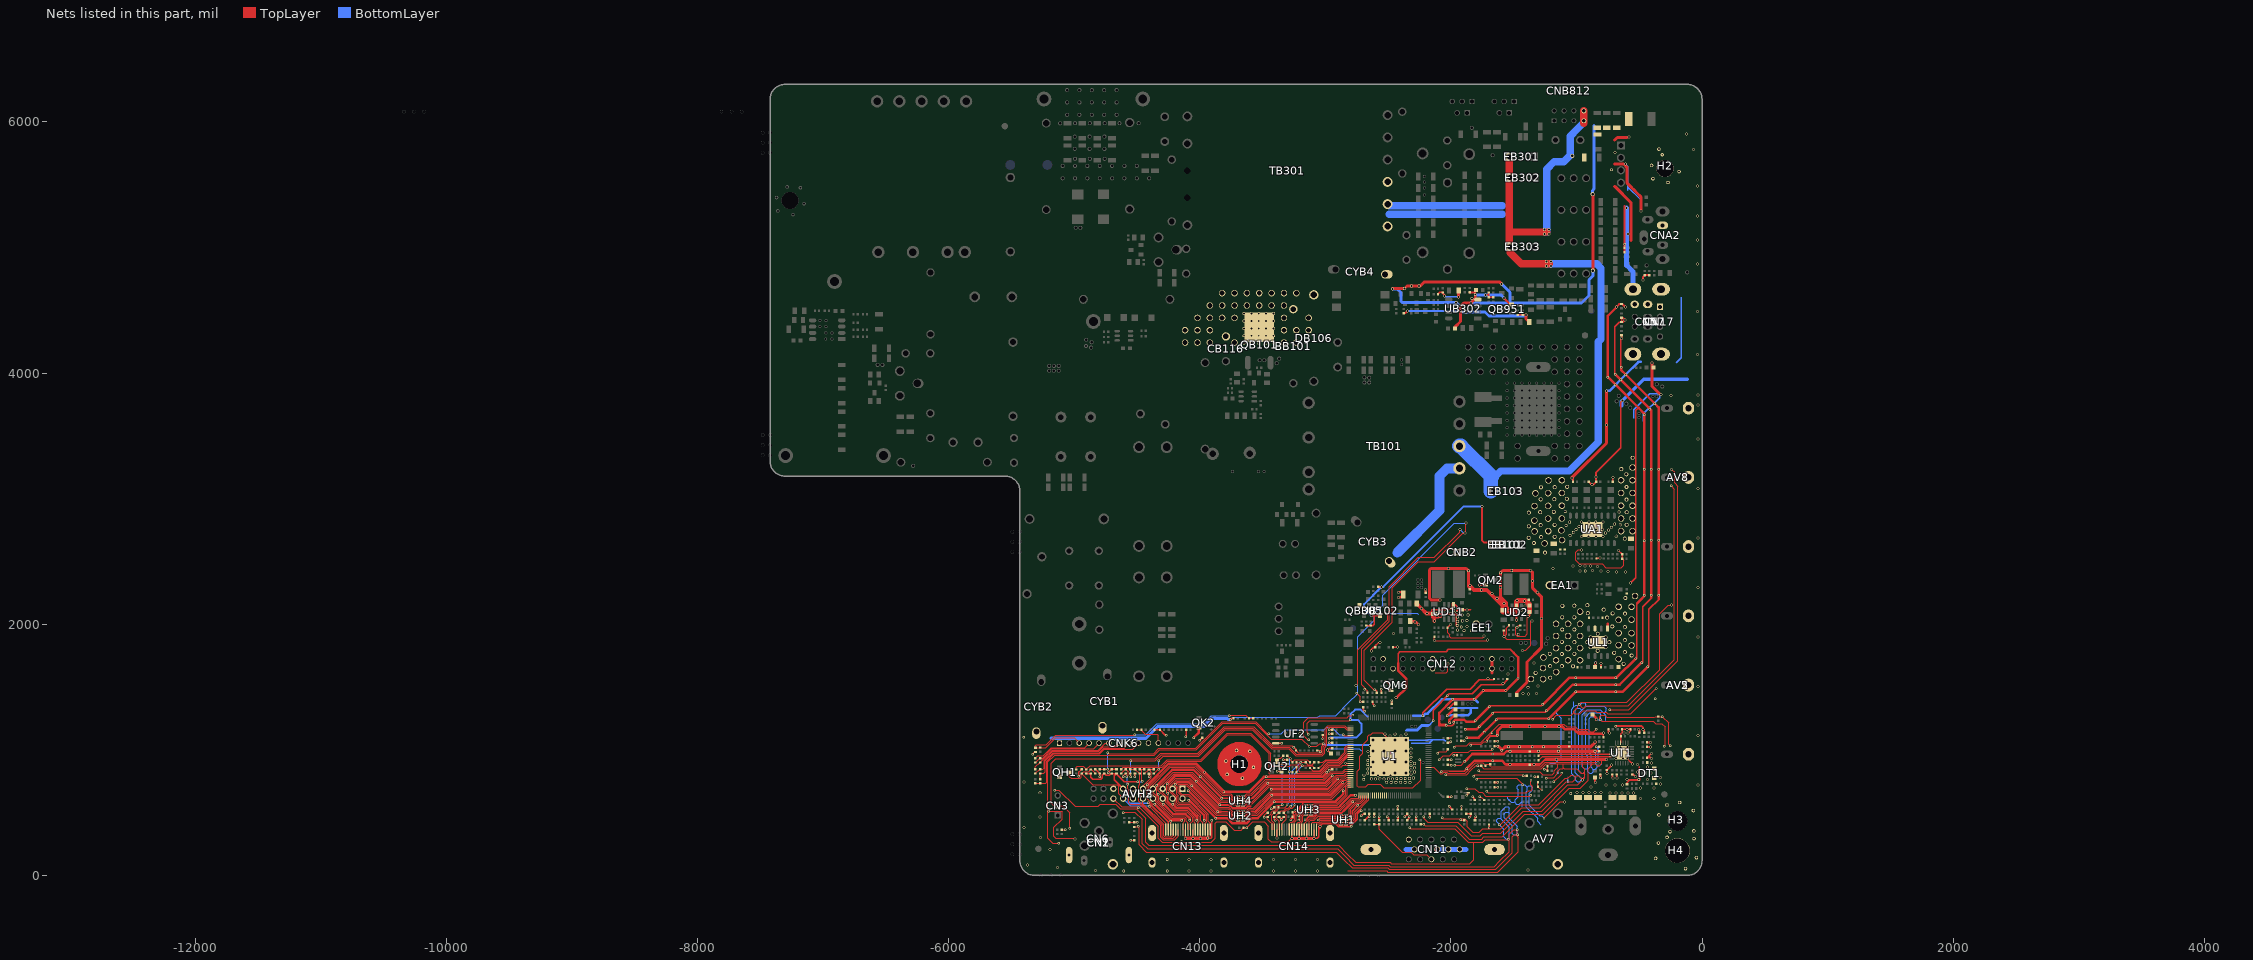
[diagram p0: the nets of this part, all layers, seen from the top]
# Altium PCB MISC84277.PcbDoc (part 10 of 15)
Units mil, origin at the board's own origin, x right, y up, seen from the top; angles counter-clockwise.
Board outline 7422.08 x 6299.21 mil, 2 copper layers (TopLayer, BottomLayer), stack 61.855 mil thick; 709 components, 395 nets, 2812 pads, 811 vias.

## Via types
v1: diameter 23.62, hole 15.75, TopLayer to BottomLayer, tented both sides, 437 vias
v2: diameter 19.68, hole 11.81, TopLayer to BottomLayer, tented both sides, 353 vias
v3: diameter 31.5, hole 23.62, TopLayer to BottomLayer, tented both sides, 16 vias
v4: diameter 31.5, hole 19.68, TopLayer to BottomLayer, tented both sides, 4 vias
v5: diameter 17.72, hole 9.84, TopLayer to BottomLayer, tented both sides, 1 vias

## Nets (pads, with @x,y where several pads share a name; then routed paths per layer and width w, separated by ;. In a path a pad name is that pad's centre, name@x,y a point inside that pad or via, vN(x,y) a via of type N, cw(c..) or ccw(c..) an arc to the next point about the centre after c; other vN are vias at no path point) (continued)
GND: (continued)
  other v1: -4606,34 -4259.5,34.5 -4085,34.5 -3910.5,34.5 -3413.04,34.5 -3238.54,34.5 -3064.04,34.5 -4829.1,37.25 -1387,41.5 -5132.2,62.6 -5372.8,82.7 -4259.5,124.5 -4085,124.5 -3910.5,124.5 -3413.04,124.5 -3238.54,124.5 -3064.04,124.5 -5194.2,204.1 -5268.5,300.8 -5400.94,382.6 -3043,388 -5271.8,463.9 -490.09,612.91 -382.59,612.91 -1046,652.26 -731.84,657.41 -685.09,657.41 -638.34,657.41 -591.59,657.41 -544.84,657.41 -5273.2,657.8 -994.84,658.91 -947.76,658.91 -900.67,658.91 -853.59,658.91 -806.5,658.91 -490.09,695.91 -382.59,695.91 -885,704.26 -33,718.5 -765.37,721.41 -694.12,721.41 -634.12,721.41 -330.5,727.76 -5400.94,743.7 -597.5,762.26 -435.12,763.41 -504.5,764.26 -332.5,777.76 -2582.1,795.6 -2482.7,796.2 -408.12,813.91 -513.5,824.76 -433.62,862.41 -1531,884.53 -1339,884.53 -513.12,884.41 -403.62,893.41 -1158,922.98 -685.18,930.04 -594.64,930.04 -628.9,931.02 -684.19,964.29 -595.63,986.33 -2662,987.1 -1302,988.47 -1142.5,988.47 -650.94,1019.59 -685.18,1020.59 -594.64,1020.59 -410.62,1021.41 -1541.4,1024.26 -1453.5,1024.26 -1352.5,1024.26 -1264.5,1024.26 -1140,1024.26 -2645.1,1034 -409.62,1059.41 -852.1,1063.1 -2399.4,1109.6 -2485.4,1110.4 -33,1112.2 -3204,1130 -3316,1134 -1526,1184.26 -1373,1184.26 -1252,1184.26 -841.6,1239.8 -1381,1445 -1426,1449 -1320,1450 -1386,1498 -33,1505.9 -1307,1509 -1585,1527 -1705,1568 -1544.11,1601.81 -1338,1691 -2634,1786 -33,1899.6 -1464,1917 -2458,1928 -1918,1979 -1872.05,1980.31 -1478,2033 -1280,2047 -1465,2082 -1504,2087 -2056,2088 -1951,2092 -1438,2108 -1532,2110 -1874,2115 -1409.26,2146.29 -1413.7,2184.95 -1474.71,2190.09 -1632.4,2204.1 -1672.2,2244.35 -1312.21,2251.54 -1758.7,2273.55 -1605,2292 -33,2293.3 -1352,2345 -682,2417 -611,2417 -748,2419 -930.5,2423.5 -973.3,2424.1 -806,2424 -872.9,2426.4 -1516,2428 -1187.1,2443.5 -833,2461 -932.9,2463.8 -1027,2465 -887.2,2465.6 -974,2466 -33,2687 -903,2697 -846,2697 -789,2697 -960,2699 -953.02,2754.94 -902.36,2754.94 -845.67,2754.94 -795.02,2754.94 -791,2813 -902,2814 -847,2814 -962,2815 -33,3080.7 -843.73,3171 -33,3474.41 -33,3747 -249,3823 -33,3824 -329,3829.5 -35.5,4146.5 -35.5,4489.5 -35.5,4868 -35.5,5059.25 -590.7,5108.6 -35.5,5250.5 -35.5,5491.5 -722.44,5619.47 -692.1,5758.6 -69,5779.5 -583.6,5881.4 -124,5906
  other v2: -4082.1,437.9 -3906.6,437.9 -4412.5,643.2 -4330.2,644.1 -4255.8,652.6 -4063.13,714.64 -1181,746 -4028.87,749.68 -3996.08,786.19 -3962.9,822.3 -1669,914.5 -1977,958 -1669,966.5 -3129.1,1026.27 -2971,1055 -1628,1069 -5400.94,1099.2 -2971,1127 -1735.14,1141.64 -1773.12,1184.27 -2038,1197 -1806,1233 -1694.53,1343.47 -373.4,1407.1 -689,1460.84 -2688,1482 -1007,1517.84 -689,1517.84 -1466.06,1570.27 -1007,1574.84 -689,1574.84 -433.33,1661.23 -481.87,1693.31 -528.64,1727.15 -2519,2088.94 -461,2230 -404,2230 -347,2230 -461,2666 -404,2667 -347,2667 -461,3236 -404,3236 -347,3236 -461,3670
  other v3: -2620.6,815.53 -2534.71,815.53 -2444.16,815.53 -2358.3,815.53 -2620.6,901.4 -2534.71,901.4 -2444.16,901.4 -2358.3,901.4 -2620.6,991.95 -2534.71,991.95 -2444.16,991.95 -2358.3,991.95 -2534.71,1077.82 -2444.16,1077.82
  other v4: -887.06,1816.63 -768.94,1816.63 -887.06,1895.37 -768.94,1895.37
H: BB101.1 CB116.2 DB106.A pad.VIA5@-3133.02,4341.45 pad.VIA5@-3133.02,4439.87 pad.VIA5@-3231.44,4243.02 pad.VIA5@-3231.44,4341.45 pad.VIA5@-3231.44,4636.72 pad.VIA5@-3329.86,4636.72 pad.VIA5@-3329.87,4243.02 pad.VIA5@-3329.87,4341.45 pad.VIA5@-3329.87,4439.87 pad.VIA5@-3329.87,4538.3 pad.VIA5@-3412.61,4238.33 pad.VIA5@-3412.61,4297.38 pad.VIA5@-3412.61,4356.44 pad.VIA5@-3412.61,4415.49 pad.VIA5@-3412.61,4474.55 pad.VIA5@-3428.29,4538.3 pad.VIA5@-3428.29,4636.72 pad.VIA5@-3471.66,4238.33 pad.VIA5@-3471.66,4297.38 pad.VIA5@-3471.66,4356.44 pad.VIA5@-3471.66,4415.49 pad.VIA5@-3471.66,4474.55 pad.VIA5@-3526.72,4538.3 pad.VIA5@-3526.72,4636.72 pad.VIA5@-3530.72,4238.33 pad.VIA5@-3530.72,4297.38 pad.VIA5@-3530.72,4356.44 pad.VIA5@-3530.72,4415.49 pad.VIA5@-3530.72,4474.55 pad.VIA5@-3589.77,4238.33 pad.VIA5@-3589.77,4297.38 pad.VIA5@-3589.77,4356.44 pad.VIA5@-3589.77,4415.49 pad.VIA5@-3589.77,4474.55 pad.VIA5@-3625.14,4538.3 pad.VIA5@-3625.14,4636.72 pad.VIA5@-3648.83,4238.33 pad.VIA5@-3648.83,4297.38 pad.VIA5@-3648.83,4356.44 pad.VIA5@-3648.83,4415.49 pad.VIA5@-3648.83,4474.55 pad.VIA5@-3723.57,4243.02 pad.VIA5@-3723.57,4439.87 pad.VIA5@-3723.57,4538.3 pad.VIA5@-3723.57,4636.72 pad.VIA5@-3821.99,4439.87 pad.VIA5@-3821.99,4538.3 pad.VIA5@-3821.99,4636.72 pad.VIA5@-3920.42,4243.02 pad.VIA5@-3920.42,4341.45 pad.VIA5@-3920.42,4439.87 pad.VIA5@-3920.42,4538.3 pad.VIA5@-4018.84,4243.02 pad.VIA5@-4018.84,4341.45 pad.VIA5@-4018.84,4439.88 pad.VIA5@-4117.27,4243.02 pad.VIA5@-4117.27,4341.45 QB101.D
HDMI1_5V: CH9.2 CN14.18 DH2.K RH8.2 RH9.2 RH14.2 RH15.1 | length 939.7
  TopLayer w8: CH9.2@-3412,498.73 -3412,495.03 -3426.84,480.19 -3426.84,434.84 -3405.51,413.51 CN14.18@-3405.51,398 ; CH9.2@-3408,498.73 -3402.75,498.73 -3376.6,524.88 -3376.6,537.97 DH2.K@-3373.17,541.4 ; CN14.18@-3405.51,364.62 CN14.18@-3405.51,398 ; CN14.18@-3405.51,411.51 CN14.18@-3405.51,398 ; DH2.K@-3369.27,538 -3325.26,538 -3317.74,545.52 -3317.68,545.52 -3305.8,557.4 v2(-3305.8,561.7) ; RH14.2@-3302.97,953.07 v2(-3277.9,928) -3277.9,915.8 RH9.2@-3263.03,899.9 -3242.49,920.44 -3143.51,920.44 RH8.2@-3122.97,899.9 ; v2(-3287.8,824) -3264.03,824 RH15.1@-3263.03,823
  BottomLayer w8: v2(-3305.8,561.7) -3282.47,585.03 -3282.47,796.2 ; -3282.47,807.47 -3282.47,796.2 ; v2(-3277.9,928) -3278.5,928 -3282.47,924.03 -3282.47,796.2
HDMI1_HPDIN: RH15.2 RH16.2 U1.113 | length 528.2
  TopLayer w6: RH15.2@-3235.27,823 -3225.1,812.84 -3036.51,812.84 -2971.35,878 -2885,878 -2824.2,938.8 U1.113@-2800.46,938.8 ; RH15.2@-3229.57,823 RH16.2@-3229.57,860
HDMI1_RX0_N: CN14.9 U1.1 UH3.3 UH3.6 | length 665.4
  TopLayer w7: CN14.9@-3228.35,364.62 -3228.35,408.29 -3214.3,422.34 -3205.76,422.34 -3192.84,435.26 -3192.84,475.03 -3166.46,501.41 UH3.3@-3154.64,501.41 UH3.6@-3113.7,501.41 -3098.06,501.41 -3074.14,525.34 -2885.26,525.34 -2795.59,615 -2738,615 -2733.53,619.47 U1.1@-2733.53,635.65
HDMI1_RX0_P: CN14.7 U1.2 UH3.4 UH3.5 | length 655.7
  TopLayer w7: CN14.7@-3188.98,364.62 -3190.53,366.17 -3190.53,420.6 -3180.84,430.29 -3180.84,470.06 -3169.17,481.73 UH3.4@-3154.64,481.73 UH3.5@-3113.7,481.73 -3100.78,481.73 -3069.17,513.34 -2880.29,513.34 -2790.62,603 -2726.54,603 -2717.79,611.76 U1.2@-2717.79,635.65
HDMI1_RX1_N: CN14.6 U1.3 UH1.1 UH1.8 | length 667
  TopLayer w7: CN14.6@-3168.04,364.62 -3168.04,409.54 -3125.56,452.03 -3092.3,452.03 -3062.99,481.34 -2937.1,481.34 ; -2912.7,481.34 -2937.1,481.34 ; UH1.1@-2878.24,481.34 -2937.1,481.34 ; UH1.1@-2875.97,480.67 UH1.8@-2835.03,480.67 -2820.13,480.67 -2811.7,489.1 -2811.7,529.6 -2754.3,587 -2722.97,587 -2702.04,607.93 U1.3@-2702.04,635.65
HDMI1_RX1_P: CN14.4 U1.4 UH1.2 UH1.7 | length 640.2
  TopLayer w7: CN14.4@-3128.67,364.62 -3128.67,429.36 -3118,440.03 -3087.33,440.03 -3058.02,469.34 -2901.07,469.34 -2892.72,460.98 UH1.2@-2875.97,460.98 UH1.7@-2835.03,460.98 -2822.84,460.98 -2799.7,484.13 -2799.7,524.63 -2749.33,575 -2718,575 -2686.29,606.71 U1.4@-2686.29,635.65
HDMI1_RX2_N: CN14.3 U1.5 UH1.3 UH1.6 | length 650.7
  TopLayer w7: CN14.3@-3108.99,364.62 -3108.99,414.65 -3101.31,422.34 -3050.56,422.34 -3035.56,437.34 -2925.2,437.34 ; -2912.7,437.34 -2925.2,437.34 ; U1.5@-2670.54,635.65 -2670.54,601.68 -2770.9,501.32 -2770.9,458.16 -2807.44,421.61 UH1.6@-2835.03,421.61 UH1.3@-2875.97,421.61 -2892.75,421.61 -2908.47,437.34 -2925.2,437.34
HDMI1_RX2_P: CN14.1 U1.6 UH1.4 UH1.5 | length 615.4
  TopLayer w7: CN14.1@-3069.62,364.62 -3069.62,403.97 -3063.25,410.34 -3045.59,410.34 -3030.59,425.34 -2913.44,425.34 -2890.04,401.93 UH1.4@-2875.97,401.93 UH1.5@-2835.03,401.93 -2822.09,401.93 -2814.4,409.61 -2802.47,409.61 -2758.9,453.19 -2758.9,496.35 -2654.79,600.46 U1.6@-2654.79,635.65
HDMI1_RXC_N: CN14.12 U1.127 UH3.1 UH3.8 | length 720.1
  TopLayer w7: CN14.12@-3286.15,364.62 -3286.15,413.85 -3277.35,422.65 -3264.98,422.65 -3243.74,443.89 -3243.74,484.22 -3167.49,560.47 UH3.1@-3154.64,560.47 UH3.8@-3113.7,560.47 -3097.7,560.47 -3088.83,569.34 -2910.55,569.34 -2836,643.89 -2836,704.34 -2822.01,718.33 U1.127@-2800.46,718.33
HDMI1_RXC_P: CN14.10 U1.128 UH3.2 UH3.7 | length 677.2
  TopLayer w7: CN14.10@-3248.03,364.62 -3248.03,422.63 -3231.74,438.92 -3231.74,479.25 -3170.21,540.79 UH3.2@-3154.64,540.79 UH3.7@-3116.83,540.79 ; UH3.7@-3113.7,540.79 -3100.41,540.79 -3083.86,557.34 -2905.58,557.34 -2824,638.92 -2824,697 -2818.42,702.58 U1.128@-2800.46,702.58 U1.128@-2799.36,702.58
HDMI1_SCL: RH10.1 U1.108 | length 343.8
  TopLayer w6: RH10.1@-3055.67,855.1 -3044.77,866 -3037.46,866 -2992.46,911 -2898.67,911 -2834,975.67 -2834,1012.06 -2828.51,1017.54 U1.108@-2800.46,1017.54
HDMI1_SCL/: CN14.15 DH6.K RH9.1 RH10.2 | length 766.7
  TopLayer w5: RH9.1@-3226.43,896.76 -3216,896.76 -3191.67,872.44 v2(-3183.2,872.44) -3106.47,872.44 RH10.2@-3089.13,855.1
  TopLayer w6: CN14.15@-3346.46,364.62 -3346.46,412.54 -3313.17,445.83 -3313.17,477.44 -3332,496.27 DH6.K@-3332,498.73 ; DH6.K@-3329.27,498.73 DH6.K@-3332,498.73 ; v2(-3246,562.9) -3246,553.4 -3265.88,533.52 -3280.69,533.52 -3291.69,522.52 -3308.21,522.52 DH6.K@-3332,498.73
  BottomLayer w6: v2(-3246,562.9) -3246,809.64 v2(-3183.2,872.44)
HDMI1_SDA: RH11.1 U1.107 | length 332.6
  TopLayer w6: RH11.1@-3056.1,899 -3020.01,899 -2997.01,922 -2903.23,922 -2845,980.23 -2845,1016.61 -2828.32,1033.29 U1.107@-2800.46,1033.29
HDMI1_SDA/: CN14.16 DH7.K RH8.1 RH11.2 | length 797.5
  TopLayer w5: v2@-3194.61,899.9 RH8.1@-3156.43,899.9 ; -3181.3,899.9 RH8.1@-3156.43,899.9 ; RH8.1@-3156.83,900.3 RH8.1@-3156.43,899.9 ; RH11.2@-3089.13,899.6 -3106.29,882.44 -3138.97,882.44 RH8.1@-3156.43,899.9
  TopLayer w6: DH7.K@-3370,498.73 DH7.K@-3368.27,498.73 ; CN14.16@-3366.14,364.62 -3366.14,430.14 -3390.16,454.16 -3390.16,476.84 DH7.K@-3368.27,498.73 ; v2(-3275.9,551.4) -3278.37,551.4 -3296.25,533.52 -3312.76,533.52 -3330.7,515.59 -3350.31,515.59 -3367.17,498.73 DH7.K@-3368.27,498.73
  BottomLayer w6: v2(-3275.9,551.4) -3264.63,562.67 -3264.63,833.28 v2(-3196.31,901.6)
HDMI2_CLKN: U1.8
HDMI2_CLKP: U1.9@-2607.55,635.65
HDMI2_HPDIN: U1.114
HDMI2_RX0N: U1.10
HDMI2_RX0P: U1.11
HDMI2_RX1N: U1.12
HDMI2_RX1P: U1.13
HDMI2_RX2N: U1.14
HDMI2_RX2P: U1.15
HDMI2_SCL: U1.110
HDMI2_SDA: U1.109
HDMI3_5V: AVH2.13 AVH3.13 CH3.2 CN13.18 DH8.K RH1.2 RH2.2 RH5.2 RH6.1 RH56.2 | length 1451.9
  TopLayer w8: RH1.2@-4479.2,844.91 -4460,844.91 ; v2@-4460.64,748.96 -4460.64,780.8 ; v2(-4459.6,749) -4460.64,750.04 -4460.64,780.8 ; RH2.2@-4441.8,844.91 -4460,844.91 ; -4460.64,780.8 -4460.64,844.27 -4460,844.91
  TopLayer w10: RH6.1@-4904,810.17 -4903.5,810.67 RH5.2@-4867.9,810.67 -4867.9,780.4 -4852.26,764.76 -4787.28,764.76 -4775.66,776.38 -4775.66,795.51 RH56.2@-4759.7,811.47 -4745.39,797.16 -4721.68,797.16 -4707.77,811.07 DH8.K@-4664.5,811.07 ; AVH2.13@-4610.26,689.7 -4610.26,690.83 -4679.9,760.48 -4679.9,794.34 -4664.5,809.74 -4601.36,746.6 -4553.5,746.6 ; -4544.6,746.6 -4553.5,746.6 ; v2@-4490.5,746.6 -4553.5,746.6 ; v2(-4412.5,578.9) -4405.62,578.9 -4251.97,425.25 CN13.18@-4251.97,364.62
  BottomLayer w8: v2(-4495.4,746) -4462.6,746 v2(-4459.6,749)
  BottomLayer w10: AVH2.13@-4610.26,689.7 -4570.3,649.74 -4570.3,589.8 -4556.46,575.96 -4415.44,575.96 v2(-4412.5,578.9)
HDMI3_CLKN: AVH2.8 AVH3.8 CN13.12 U1.119 UH4.1 UH4.8 | length 2384.3
  TopLayer w7: CN13.12@-4133.86,364.62 -4133.86,415.54 -4119.1,430.3 -4119.1,446.9 -4128.6,456.4 -4222.37,456.4 -4351.4,585.43 -4351.4,619.23 -4358.58,626.41 -4407.8,675.63 -4407.8,703.97 -4240.07,871.7 -4038.46,871.7 -3815.32,648.55 -3754.53,648.55 -3737.66,631.69 UH4.1@-3695.54,631.69 UH4.8@-3654.6,631.69 -3641.41,631.69 -3624.55,648.55 -3589.95,648.55 -3473.16,765.34 -3016.84,765.34 -2957.17,825 -2861,825 -2841.69,844.31 U1.119@-2800.46,844.31
HDMI3_CLKP: AVH2.7 AVH3.7 CN13.10 U1.120 UH4.2 UH4.7 | length 2370.3
  TopLayer w7: CN13.10@-4094.49,364.62 -4094.49,417.19 -4107.1,429.8 -4107.1,455.26 -4120.24,468.4 -4217.4,468.4 -4339.4,590.4 -4339.4,624.2 -4395.8,680.6 -4395.8,699 -4235.1,859.7 -4043.43,859.7 -3820.29,636.55 -3759.5,636.55 -3742.63,619.69 -3715.6,619.69 -3707.91,612 UH4.2@-3695.54,612 UH4.7@-3654.6,612 -3644.13,612 -3619.58,636.55 -3584.98,636.55 -3468.19,753.34 -3011.87,753.34 -2952.2,813 -2856.03,813 -2840.46,828.57 U1.120@-2800.46,828.57
HDMI3_HPDIN: RH6.2 RH7.2 U1.112 | length 2595.8
  TopLayer w6: RH7.2@-4985.1,843.63 -4985.1,859.3 -4976.8,867.6 -4927.97,867.6 RH6.2@-4904,843.63 -4874.54,873.09 -4305.85,873.09 -4259.75,919.2 -3994.16,919.2 -3783.2,1130.16 -3594.32,1130.16 -3434.73,970.56 -3434.73,883.43 -3419.89,868.58 -3284.46,868.58 -3274.05,879 -3218.55,879 -3209.3,869.75 -3209.3,830.84 -3202.3,823.84 -3041.07,823.84 -2975.91,889 -2889.56,889 -2824.01,954.55 U1.112@-2800.46,954.55
HDMI3_RX0N: AVH2.6 AVH3.6 CN13.9 U1.121 UH4.3 UH4.6 | length 2294.3
  TopLayer w7: AVH2.6@-4273.13,618.73 -4272.9,618.5 -4272.9,580.97 -4197.33,505.4 -4104.91,505.4 -4057.1,457.59 -4057.1,431.2 -4074.81,413.49 CN13.9@-4074.81,364.62 ; AVH2.6@-4272.9,618.97 -4280.09,626.16 -4329.23,675.3 -4329.23,703.84 -4319.29,713.79 -4210.37,822.7 -4058.76,822.7 -3831.61,595.55 -3756.69,595.55 -3733.76,572.63 UH4.3@-3695.54,572.63 UH4.6@-3654.6,572.63 -3639.04,572.63 -3630.95,580.72 -3588.49,580.72 -3452.87,716.34 -2996.54,716.34 -2914.88,798 -2850,798 -2835.18,812.82 U1.121@-2800.46,812.82
HDMI3_RX0P: AVH2.5 AVH3.5 CN13.7 U1.122 UH4.4 UH4.5 | length 2276.1
  TopLayer w7: CN13.7@-4035.44,364.62 -4035.44,414.74 -4045.1,424.4 -4045.1,462.56 -4099.94,517.4 -4192.36,517.4 -4260.9,585.94 -4260.9,623.94 -4310.98,674.02 -4317.23,680.27 -4317.23,698.87 -4205.4,810.7 -4063.73,810.7 -3836.58,583.55 -3761.66,583.55 -3738.73,560.63 -3717,560.63 -3709.31,552.94 UH4.4@-3695.54,552.94 UH4.5@-3654.6,552.94 -3641.75,552.94 -3625.98,568.72 -3583.52,568.72 -3447.9,704.34 -2991.57,704.34 -2909.91,786 -2845.03,786 -2833.96,797.07 U1.122@-2800.46,797.07
HDMI3_RX1N: AVH2.4 AVH3.4 CN13.6 U1.123 UH2.1 UH2.8 | length 2205.9
  TopLayer w7: CN13.6@-4015.75,364.62 -4015.75,420.05 -4002.9,432.9 -4002.9,472.69 -4084.61,554.4 -4177.04,554.4 -4194.7,572.06 -4194.7,619.83 -4201.19,626.32 -4251.3,676.43 -4251.3,712.47 -4190.07,773.7 -4079.06,773.7 -3847.91,542.55 -3770.15,542.55 -3740.14,512.54 UH2.1@-3695.54,512.54 UH2.8@-3654.6,512.54 -3631.21,512.54 -3610.2,533.55 -3574.58,533.55 -3440.8,667.34 -2976.25,667.34 -2873.5,770.08 -2839.94,770.08 -2828.7,781.32 U1.123@-2800.46,781.32
HDMI3_RX1P: AVH2.3 AVH3.3 CN13.4 U1.124 UH2.2 UH2.7 | length 2191.5
  TopLayer w7: CN13.4@-3976.38,364.62 -3976.38,420.28 -3990.9,434.8 -3990.9,477.66 -4079.64,566.4 -4172.07,566.4 -4182.7,577.03 -4182.7,624.8 -4239.3,681.4 -4239.3,707.5 -4185.1,761.7 -4084.03,761.7 -3852.88,530.55 -3775.12,530.55 -3745.11,500.54 -3717,500.54 -3709.31,492.86 UH2.2@-3695.54,492.86 UH2.7@-3654.6,492.86 -3633.93,492.86 -3605.23,521.55 -3569.61,521.55 -3435.83,655.34 -2971.28,655.34 -2868.53,758.08 -2834.97,758.08 -2827.47,765.57 U1.124@-2800.46,765.57
HDMI3_RX2N: AVH2.2 AVH3.2 CN13.3 U1.125 UH2.3 UH2.6 | length 2094.7
  TopLayer w7: CN13.3@-3956.7,364.62 -3956.7,415.8 -3944.2,428.3 -3944.2,483.28 -4093.52,632.6 -4147.8,632.6 -4172.1,656.9 -4172.1,718.77 -4166.17,724.7 -4099.35,724.7 -3864.2,489.55 -3772.31,489.55 -3736.24,453.49 UH2.3@-3695.54,453.49 -3633.32,453.49 -3597.26,489.55 -3549.28,489.55 -3420.5,618.34 -2955.95,618.34 -2824.46,749.83 U1.125@-2800.46,749.83
HDMI3_RX2P: AVH2.1 AVH3.1 CN13.1 U1.126 UH2.4 UH2.5 | length 2078
  TopLayer w7: CN13.1@-3917.33,364.62 -3917.33,415.82 -3932.2,430.7 -3932.2,488.25 -4088.55,644.6 -4142.83,644.6 -4160.1,661.87 -4160.1,709.4 -4156.8,712.7 -4104.32,712.7 -3869.17,477.55 -3777.28,477.55 -3741.21,441.49 -3715.3,441.49 -3707.61,433.8 UH2.4@-3695.54,433.8 UH2.5@-3654.6,433.8 -3636.04,433.8 -3592.29,477.55 -3544.31,477.55 -3415.53,606.34 -2950.98,606.34 -2823.24,734.08 U1.126@-2800.46,734.08
HDMI3_SCL: RH3.1 U1.99 | length 2040.8
  TopLayer w6: RH3.1@-4362.94,811.44 -4329.48,844.91 v2(-4328.82,844.25) ; v2(-4328.8,911) -4289.6,950.2 -4007.7,950.2 -3796.74,1161.16 -3581.48,1161.16 -3427.92,1007.6 -3292.88,1007.6 -3237.72,952.44 -3025.86,952.44 -3006.91,971.39 -3006.91,1017.89 -2988.84,1035.96 -2988.84,1166.8 -2974.85,1180.8 -2850.8,1180.8 -2829.27,1159.27 U1.99@-2800.46,1159.27
  BottomLayer w6: v2(-4328.82,844.25) v2@-4328.82,910.95
HDMI3_SCL/: AVH2.9 AVH3.9 CN13.15 DH4.K RH2.1 RH3.2 | length 956
  TopLayer w6: RH2.1@-4441.8,811.44 -4438.66,811.44 -4407.27,842.83 DH4.K@-4404.7,842.83 ; DH4.K@-4409.72,844.91 DH4.K@-4404.7,844.91 ; -4385.04,816.08 -4385.04,778.35 ; RH3.2@-4373.5,844.91 DH4.K@-4404.7,844.91 ; CN13.15@-4192.92,364.62 -4192.92,315.48 -4212.6,295.8 -4285.66,295.8 -4299.1,309.24 -4299.1,402.94 -4485.78,589.62 -4485.78,624.63 -4452.78,657.63 AVH3.9@-4452.78,689.7 -4452.78,710.61 -4385.04,778.35 ; DH4.K@-4404.7,842.83 -4404.7,841.6 -4385.04,821.94 -4385.04,778.35 ; DH4.K@-4404.7,842.83 DH4.K@-4404.7,844.91
HDMI3_SDA: RH4.1 U1.98 | length 2303.4
  TopLayer w6: RH4.1@-4553.4,811.44 -4551,809.04 v2(-4551,784.9) ; v2(-4549.6,911) -4355.1,911 -4304.9,961.2 -4012.3,961.2 -3801.35,1172.16 -3576.92,1172.16 -3423.37,1018.6 -3288.32,1018.6 -3233.17,963.44 -3030.41,963.44 -3017.91,975.95 -3017.91,1022.45 -2999.84,1040.51 -2999.84,1171.36 -2979.4,1191.8 -2846.24,1191.8 -2829.47,1175.02 U1.98@-2800.46,1175.02
  BottomLayer w6: v2(-4551,784.9) -4551,909.6 v2(-4549.6,911)
HDMI3_SDA/: AVH2.10 AVH3.10 CN13.16 DH5.K RH1.1 RH4.2 | length 801.9
  TopLayer w6: RH4.2@-4553.4,844.91 -4553.08,845.23 DH5.K@-4516.6,845.23 -4482.81,811.44 RH1.1@-4479.9,811.44 ; v2(-4488.8,647) -4485.78,650.02 -4485.78,715.6 -4477.5,723.88 RH1.1@-4477.5,811.44 ; AVH2.10@-4452.78,610.96 -4452.78,572.18 -4288.1,407.5 -4288.1,313.8 -4281.1,306.8 -4225.2,306.8 -4212.6,319.4 CN13.16@-4212.6,364.62
  BottomLayer w6: v2(-4488.8,647) AVH2.10@-4452.78,610.96
HDMI_ARC: CH15.1 U1.117 | length 2197.3
  TopLayer w6: CH15.1@-4627.5,844.73 -4610.14,862.09 -4301.3,862.09 -4255.19,908.2 -3989.6,908.2 -3778.64,1119.16 -3598.88,1119.16 -3448.95,969.23 -3448.95,807.9 -3442.88,801.84 -3031.96,801.84 -2967.79,866 -2870.97,866 -2861.16,875.81 U1.117@-2800.46,875.81
HDMI_ARC/: CH15.2 CN13.14 DH3.K | length 969
  TopLayer w6: CH15.2@-4627.5,811.27 -4594.44,844.33 DH3.K@-4590.4,844.33 -4571.57,825.51 -4571.57,795.48 v2(-4580.88,786.17) ; v2(-4573.2,726.7) -4573.2,690 -4566.1,682.9 -4566.1,580 -4553.2,567.1 -4478.81,567.1 -4466.85,555.13 -4310.1,398.39 -4310.1,304.69 -4290.21,284.8 -4199,284.8 -4173.23,310.57 CN13.14@-4173.23,364.62
  BottomLayer w6: v2(-4580.88,786.17) -4579.62,784.9 -4579.62,730.92 -4577.42,730.92 v2(-4573.2,726.7)
HDMI_CEC: RH13.1 U1.111 | length 387
  TopLayer w6: RH13.1@-3122.97,855.1 -3102.7,834.84 -3045.63,834.84 -2980.46,900 -2894.11,900 -2823.81,970.3 U1.111@-2800.46,970.3
HDMI_DET: RH55.1 RH56.1 U1.102 | length 2320.3
  TopLayer w6: RH55.1@-4795.5,844.83 -4733.77,844.83 v2(-4731.7,846.9) ; v2(-4731.9,974.7) -4725.04,967.84 -4368.97,967.84 -4325.61,1011.2 -4033.01,1011.2 -3822.06,1222.16 -3556.21,1222.16 -3462.1,1128.04 v2(-3450.91,1128.04) ; v2(-2858,1120) -2850.03,1112.03 U1.102@-2800.46,1112.03
  BottomLayer w6: v2(-4731.9,974.7) -4731.7,974.5 v2(-4731.7,846.9) ; v2(-3450.91,1128.04) -3352.56,1128.04 -3319.18,1161.42 -3007.58,1161.42 -2991,1178 -2949.23,1178 -2891.39,1120.16 v2@-2858.16,1120.16 ; v2@-2859,1121 v2@-2858.16,1120.16 ; v2(-2858,1120) v2@-2858.16,1120.16
HOTPLUG1: CH8.2 CN14.19 DH1.K QH2.C RH14.1 | length 817.3
  TopLayer w5: CH8.2@-3458,465.27 -3433,490.29 -3433,503.04 -3420.95,515.09 -3402.65,515.09 -3390.27,527.47 -3390.27,554.59 -3385.13,559.73 -3346.77,559.73 v2(-3343.6,562.9)
  TopLayer w6: CH8.2@-3458.73,465.27 -3462,465.27 -3462,447 -3446.26,431.26 ; v2(-3343.6,562.9) v2@-3343.6,567.84 ; v2@-3343.6,886.27 -3368.47,886.27 -3387.2,905 QH2.C@-3387.2,908.93 -3387.2,913.7 -3366.6,934.3 -3355.2,934.3 RH14.1@-3336.43,953.07 ; v2@-3341.87,886.27 DH1.K@-3304.8,886.27 ; -3329.37,886.47 DH1.K@-3304.6,886.47 DH1.K@-3304.8,886.27 ; DH1.K@-3304.6,886.27 DH1.K@-3304.8,886.27
  TopLayer w7: -3446.26,431.26 -3425.2,410.2 CN14.19@-3425.2,364.62
  BottomLayer w6: v2(-3343.6,562.9) v2(-3343.6,888.4)
HOTPLUG3: AVH2.14 AVH3.14 CH4.2 CN13.19 DH9.K QH1.C RH5.1 | length 1263.9
  TopLayer w5: QH1.C@-5038.27,819.58 -5038.27,787.07 -5024.76,773.56 -4953.44,773.56 -4945.86,781.14 -4945.86,805.81 DH9.K@-4940.9,810.77 ; CH4.2@-4831.7,811.37 -4864.47,844.13 RH5.1@-4867.9,844.13 -4885.51,826.53 -4925.14,826.53 DH9.K@-4940.9,810.77 ; AVH2.14@-4610.26,610.96 -4647.3,648.01 -4647.3,710.2 -4659.3,722.2 -4852.33,722.2 DH9.K@-4940.9,810.77 ; v2(-4404.38,549.02) -4271.66,416.29 CN13.19@-4271.66,364.62 CN13.19@-4271.66,413.57
  BottomLayer w5: AVH2.14@-4610.26,610.96 -4554.7,555.4 v2@-4409.46,555.4
HS_VGA: CN11.13 RV12.1 RV13.1 | length 592.8
  TopLayer w6: RV12.1@-2610,406.27 RV13.1@-2572,406.27 -2572,367 -2388,183 -2317,183 -2298,164 -2191.51,164 CN11.13@-2155.51,128
IFAGC: CT19.2 RT2.1 RT18.2 U1.43 | length 1650.4
  TopLayer w7: U1.43@-2155.76,860.06 U1.43@-2178.42,860.06 -2138.12,860.06 -2086.56,808.5 -2069.2,808.5 -2056.46,821.24 -2033.84,821.24 -2026.4,813.8 -1885.11,813.8 -1802.91,896 -1747.27,896 CT19.2@-1725.27,874 CT19.2@-1725.27,877.27
  TopLayer w8: CT19.2@-1725.27,874 -1716.27,883 -1686.73,883 -1686.73,869.73 -1680,863 -1286.38,863 -1247.41,901.98 -1229,901.98 ; -1238.41,901.98 -1229,901.98 ; v2(-844.59,1025.41) RT2.1@-819.09,1025.41 ; -836.72,901.98 -1229,901.98
  BottomLayer w8: v2(-844.59,1025.41) -828,1008.83 v1(-828,893.26)
IFN: RT9.2 UT1.16 | length 587.7
  TopLayer w10: -745.97,965.47 UT1.16@-720.63,965.47
  TopLayer w12: RT9.2@-1302.21,950.79 -1287.53,965.47 -745.97,965.47
IFP: RT10.2 UT1.17 | length 594.2
  TopLayer w10: -746.06,945.98 -745.86,945.78 UT1.17@-720.63,945.78
  TopLayer w12: RT10.2@-1302.21,915.79 -1272.02,945.98 -746.06,945.98
IR: CNK6.11 RK15.2 RK16.2 | length 247.9
  TopLayer w5: RK15.2@-4499.37,1160 -4471.4,1160 -4434,1122.6 -4340.4,1122.6 -4330.41,1112.61 CNK6.11@-4330.41,1053.3
K0: CNK6.9 RK6.1 RK7.1 | length 1079.3
  TopLayer w5: RK6.1@-5308.96,732.7 RK7.1@-5271.45,732.7 ; -5256.56,732.7 RK7.1@-5271.45,732.7 ; -5242.56,732.7 -5228.9,732.7 ; CNK6.9@-4487.89,1050.3 -4535.15,1003.04 -4759.88,1003.04 -4795.58,967.34 -5161.74,967.34 -5221,908.08 -5221,740.6 -5228.9,732.7 ; RK7.1@-5271.45,732.7 -5228.9,732.7
K1: CNK6.8 RK7.2 RK8.1 | length 920.5
  TopLayer w5: RK7.2@-5271.45,766.17 RK8.1@-5271.45,811.44 -5244.66,811.44 -5231,825.1 -5231,912.22 -5217.22,926.01 ; -5224.64,918.58 -5217.22,926.01 ; -5013.7,977.34 -5003.8,977.34 ; CNK6.8@-4566.63,1050.3 -4603.89,1013.04 -4764.03,1013.04 -4799.73,977.34 -5003.8,977.34 ; -5217.22,926.01 -5165.88,977.34 -5003.8,977.34
K2: CNK6.7 RK8.2 RK9.1 | length 904.8
  TopLayer w5: RK9.1@-5308.96,811.44 -5275.5,844.91 RK8.2@-5271.45,844.91 -5250.29,844.91 -5241,854.2 -5241,916.36 -5223.36,934 ; RK8.2@-5275.5,849.53 RK8.2@-5271.45,849.53 ; -5229.09,928.27 -5223.36,934 ; -4949.9,987.34 -4856.2,987.34 ; CNK6.7@-4645.37,1050.3 -4672.63,1023.04 -4768.17,1023.04 -4803.87,987.34 -4856.2,987.34 ; -5223.36,934 -5170.02,987.34 -4856.2,987.34
K3: CNK6.6 RK9.2 RK10.1 | length 718.8
  TopLayer w5: RK9.2@-5308.96,849.53 -5308.96,864.28 RK10.1@-5271.45,901.79 ; RK10.1@-5271.45,899.44 -5271.45,900.05 -5174.16,997.34 -4914.5,997.34 ; -4954.04,997.34 -4914.5,997.34 ; CNK6.6@-4724.11,1053.3 -4752.05,1053.3 -4808.01,997.34 -4914.5,997.34
K4: CNK6.5 RK10.2 RK11.1 | length 621.7
  TopLayer w5: RK11.1@-5308.96,901.79 -5304.92,901.79 -5271.45,935.26 RK10.2@-5269.1,932.9 ; RK10.2@-5271.45,932.9 RK10.2@-5269.1,932.9 ; RK10.2@-5264.8,928.6 RK10.2@-5269.1,932.9 ; -4958.18,1007.34 -4914.5,1007.34 ; CNK6.5@-4802.85,1050.3 -4845.81,1007.34 -4914.5,1007.34 ; RK10.2@-5269.1,932.9 -5252.75,932.9 -5178.31,1007.34 -4914.5,1007.34
K5: CNK6.4 RK11.2 | length 504.1
  TopLayer w5: RK11.2@-5308.96,935.26 -5292.6,951.61 -5275,951.61 ; -5258.5,951.61 -5275,951.61 ; -5141.1,1017.34 -5128.5,1017.34 ; CNK6.4@-4881.59,1050.3 -4914.55,1017.34 -5128.5,1017.34 ; -5275,951.61 -5248.18,951.61 -5182.45,1017.34 -5128.5,1017.34
K6: CNK6.3 DK1.K RK3.2 RK4.1 RK5.1 | length 2260.5
  TopLayer w5: CNK6.3@-4960.33,1053.3 -5002.13,1095.1 -5148.46,1095.1 -5225.47,1018.09 RK5.1@-5271.45,1018.09 -5273.18,1016.36 DK1.K@-5308.96,1016.36 -5308.96,1031.74 -5301.3,1039.4 -5221.9,1039.4 -5146.6,1114.7 v2@-4522.4,1114.7
  TopLayer w6: v2@-4522.4,1114.7 v2(-4518.3,1118.8) ; v2(-3764.4,1269.9) -3758.75,1275.55 -3633.82,1275.55 RK3.2@-3609.27,1251 RK4.1@-3573.73,1251
  BottomLayer w6: v2(-4518.3,1118.8) -4429.68,1118.8 -4341.28,1207.2 -3970.76,1207.2 -3907.61,1270.35 v2@-3764.4,1270.35